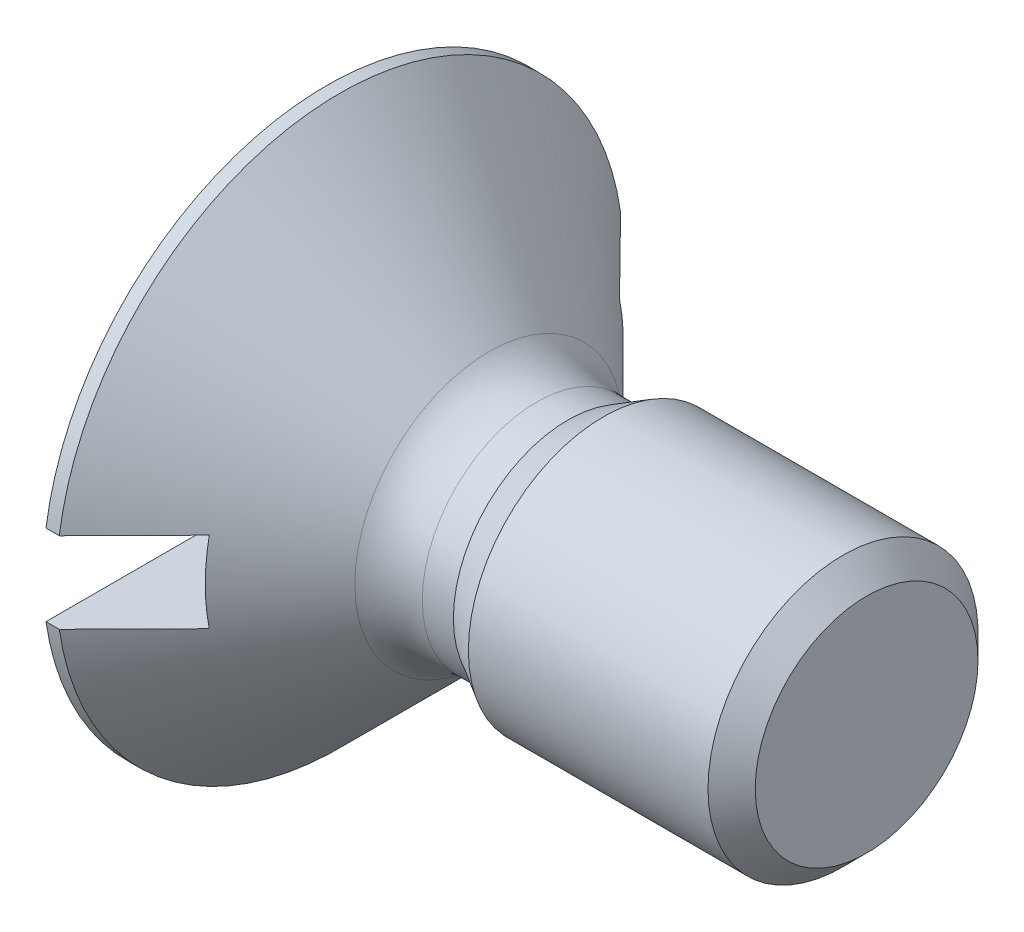
from build123d import *

# Parameters (mm, degrees)
CHAMFER1_SIZE      = 0.35
CUT_EXTRUDE1_START = -1.3
CUT_EXTRUDE1_DEPTH = 1.3


with BuildPart() as part:
    # Sketch1 → Base-Revolve (revolve)
    with BuildSketch(Plane.XY, mode=Mode.PRIVATE) as base_revolve_sk:
        with BuildLine():
            Line((0, 0), (0, 4.2))
            Line((0, 4.2), (0.1969, 4.2))
            Line((0.1969, 4.2), (2.407106781, 1.989793219))
            ThreePointArc((2.407106781, 1.989793219), (2.73153013, 1.773020467), (3.114213562, 1.6969))
            Line((3.114213562, 1.6969), (3.5750154, 1.6969))
            Line((3.5750154, 1.6969), (4.1, 2))
            Line((4.1, 2), (8, 2))
            Line((8, 2), (8, 0))
            Line((8, 0), (0, 0))
        make_face()
    revolve(base_revolve_sk.sketch.rotate(Axis((0, 0, 0), (1, 0, 0)), 90), axis=Axis((0, 0, 0), (1, 0, 0)))

    # Chamfer1
    chamfer1_edges = [part.edges().sort_by_distance(p)[0] for p in [
        (8, 0, -2),
    ]]
    chamfer(chamfer1_edges, length=CHAMFER1_SIZE)

    # Sketch3 → Cut-Extrude1 (cut)
    with BuildSketch(Plane.ZY.offset(CUT_EXTRUDE1_START)):
        with BuildLine():
            Line((-4.156921938, 0.6), (4.156921938, 0.6))
            ThreePointArc((4.156921938, 0.6), (4.2, 0), (4.156921938, -0.6))
            Line((4.156921938, -0.6), (-4.156921938, -0.6))
            ThreePointArc((-4.156921938, -0.6), (-4.2, 0), (-4.156921938, 0.6))
        make_face()
    extrude(amount=CUT_EXTRUDE1_DEPTH, mode=Mode.SUBTRACT)


solid = part.part
